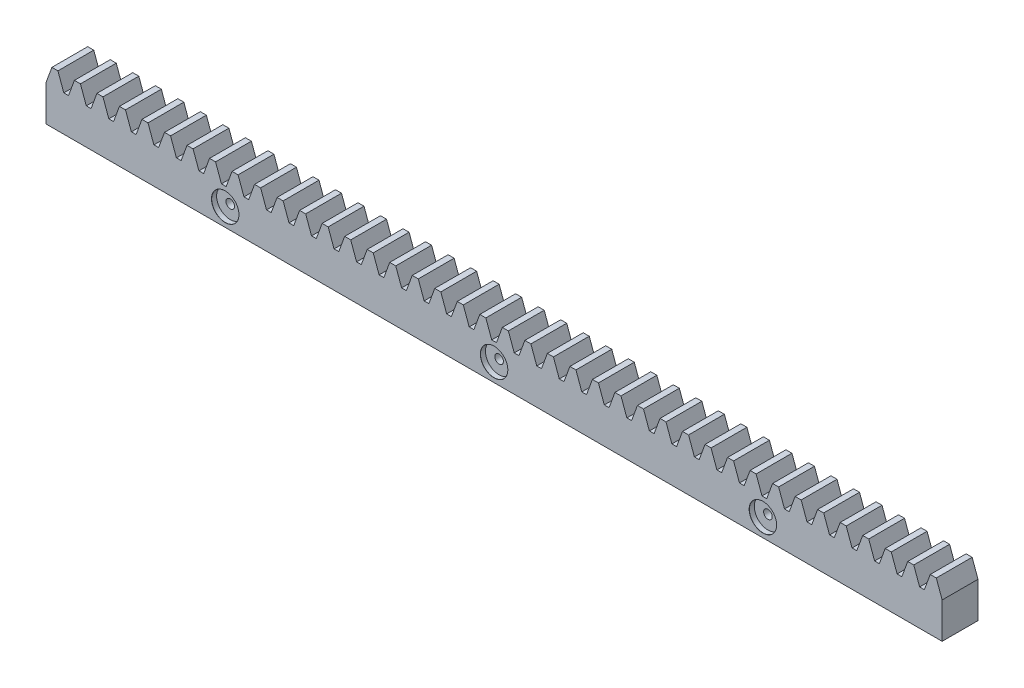
from build123d import *

# Parameters (mm, degrees)
SKETCH1_W                              = 250
SKETCH1_H                              = 10
EXTRUDE1_DEPTH                         = 10
EXTRUDE2_DEPTH                         = 10
LPATTERN1_COUNT                        = 40
LPATTERN1_PITCH                        = 6.283185307
CBORE_FOR_M2_HEX_CAP_SCREW1_AT_2_COUNT = 2
CBORE_FOR_M2_HEX_CAP_SCREW1_AT_2_PITCH = 75
CBORE_FOR_M2_HEX_CAP_SCREW1_AT_3_COUNT = 2
CBORE_FOR_M2_HEX_CAP_SCREW1_AT_3_PITCH = 150


with BuildPart() as part:
    # Sketch1 → Extrude1 (new body)
    with BuildSketch(Plane.XY):
        with Locations((125, -5)):
            Rectangle(SKETCH1_W, SKETCH1_H)
    extrude(amount=EXTRUDE1_DEPTH)

    # Sketch2 → Extrude2 (add)
    with BuildSketch(Plane.XY.offset(10)):
        Polygon((0, 0), (1.637866054, 4.5), (3.323577771, 4.5), (4.961443825, 0), align=None)
    extrude2 = extrude(amount=-EXTRUDE2_DEPTH)

    # LPattern1: Extrude2 ×40
    with Locations(*[(i * LPATTERN1_PITCH, 0, 0) for i in range(1, LPATTERN1_COUNT)]):
        add(extrude2)

    # Sketch13 → CBORE for M2 Hex Cap Screw1 (revolve, cut)
    with BuildSketch(Plane(origin=(50, -5, 10), x_dir=(0, -1, 0), z_dir=(1, 0, 0))):
        Polygon((0, 0), (0, 15.721032743), (1.2, 15), (1.2, 1.4), (3.8095, 1.4), (3.8095, 0.025), (3.8345, 0), align=None)
    cbore_for_m2_hex_cap_screw1 = revolve(axis=Axis((50, -5, 16.35), (0, 0, -1)), mode=Mode.SUBTRACT)

    # CBORE for M2 Hex Cap Screw1 at 2: CBORE for M2 Hex Cap Screw1 ×2
    with Locations(*[(i * CBORE_FOR_M2_HEX_CAP_SCREW1_AT_2_PITCH, 0, 0) for i in range(1, CBORE_FOR_M2_HEX_CAP_SCREW1_AT_2_COUNT)]):
        add(cbore_for_m2_hex_cap_screw1, mode=Mode.SUBTRACT)

    # CBORE for M2 Hex Cap Screw1 at 3: CBORE for M2 Hex Cap Screw1 ×2
    with Locations(*[(i * CBORE_FOR_M2_HEX_CAP_SCREW1_AT_3_PITCH, 0, 0) for i in range(1, CBORE_FOR_M2_HEX_CAP_SCREW1_AT_3_COUNT)]):
        add(cbore_for_m2_hex_cap_screw1, mode=Mode.SUBTRACT)


solid = part.part
